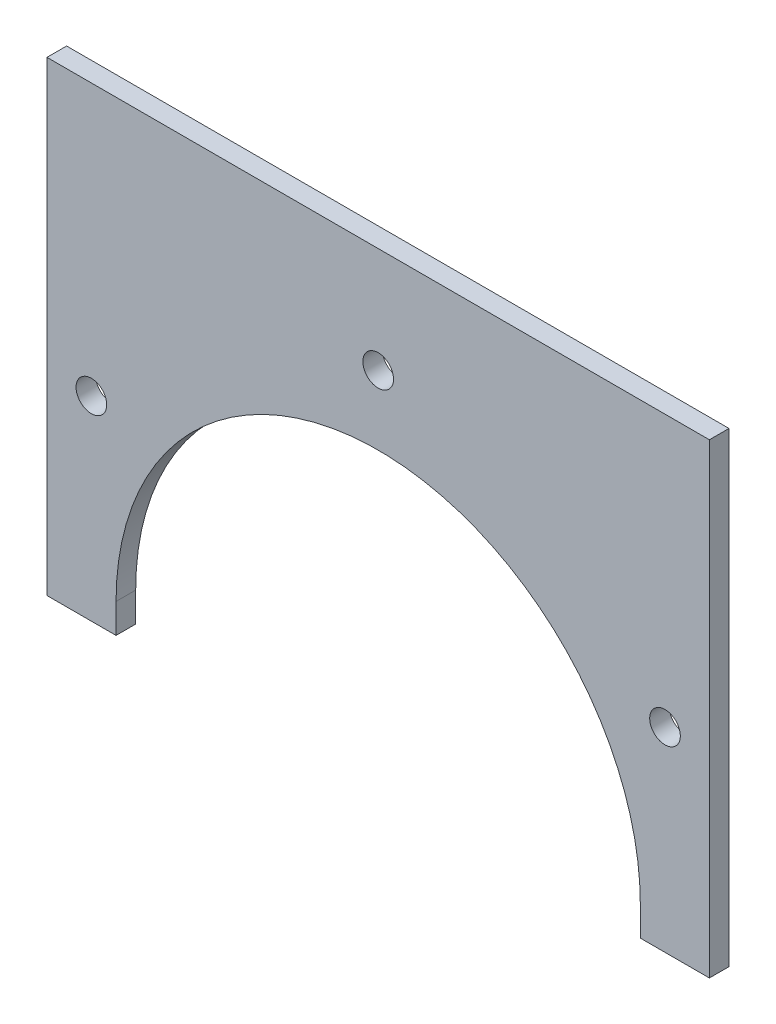
SolidWorks part; units mm, degrees
material "Q235B"
ref_plane "Front Plane" through (0, 0, 0) normal (0, 0, 1) x (1, 0, 0)
ref_plane "Top Plane" through (0, 0, 0) normal (0, 1, 0) x (1, 0, 0)
ref_plane "Right Plane" through (0, 0, 0) normal (1, 0, 0) x (0, 0, -1)
sketch "Sketch1" plane through (0, 0, 0) normal (0, 0, 1) x (-1, 0, 0)
  line L0 (-106.85, 12) -> (-135, 12)
  line L1 (106.85, 0) -> (106.85, 12)
  line L2 (-106.85, 0) -> (-106.85, 12)
  line L3 (-135, 12) -> (-135, -178)
  line L4 (-135, -178) -> (135, -178)
  line L5 (0, 0) -> (0, 75.9389) construction
  line L6 (135, 12) -> (135, -178)
  line L7 (106.85, 12) -> (135, 12)
  arc A0 (-106.85, 0) -> (106.85, 0) centre (0, 0) ccw
  dimension "D4" = 106.85
  dimension "D1" = 0
  dimension "D2" = 178
  dimension "D3" = 12
  dimension "D5" = 270
extrude "Boss-Extrude1" add sketch "Sketch1" along normal blind 8
sketch "Sketch2" plane through (0, 0, 0) normal (0, 0, -1) x (-1, 0, 0)
  circle A0 centre (-116.9134, 67.5) radius 6.25
  circle A1 centre (116.9134, 67.5) radius 6.25
  circle A2 centre (0, 135) radius 6.25
  dimension "D1" = 12.5
extrude "Cut-Extrude1" cut sketch "Sketch2" against normal through all
